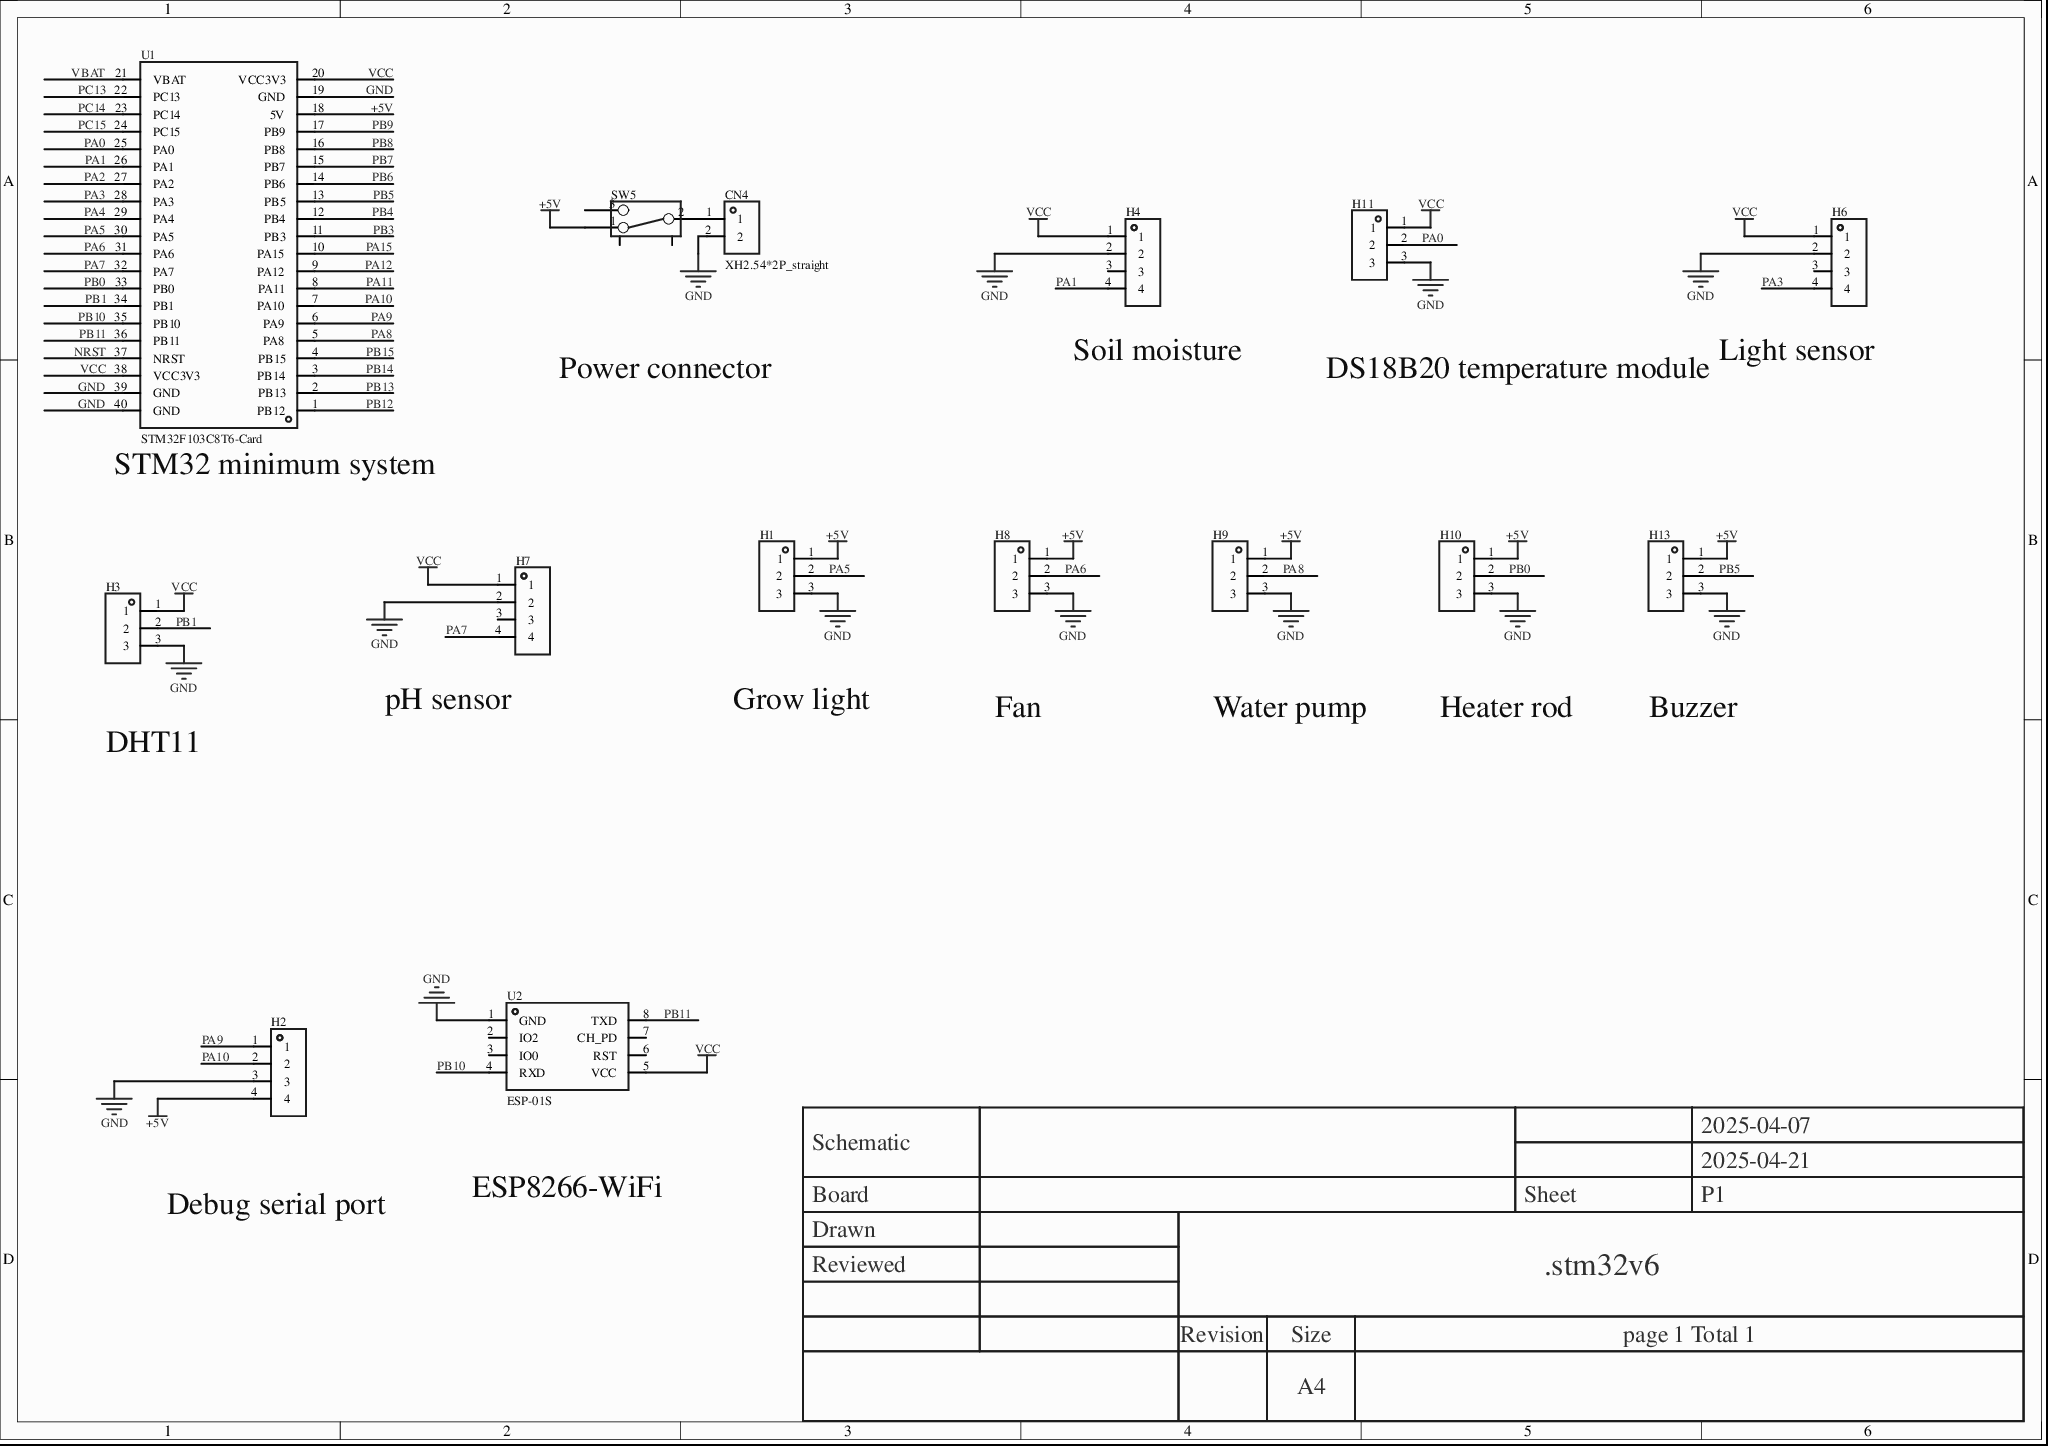
[diagram p0: MISC89003-3.schdoc]
# Altium project MISC89003-2.PrjPcb
1 sheet, 15 parts. Net scope: global (net labels, ports and power ports of the same name join across sheets).
Board file: MISC89003.pcbdoc

## Sheet MISC89003-3.schdoc
size 297 x 209 mm; Version: V1.0; @Project Name: MISC89003; @Page Count: 1; @Update Date: 2026-04-15; @Create Date: 2026-04-15; @Schematic Name: MISC89003; @Page No: 1; @Create Time: 23:22:16; @Update Time: 17:32:40; @Board Name: MISC89003

### Parts
CN4  XH2.54*2P_straight  [CONN-TH_2P-P2.50-XH2.54-2P]
H1  (no value)  [HDR-TH_3P-P2.54-V-F]
H2  (no value)  [HDR-TH_4P-P2.54-V-F]
H3  (no value)  [HDR-TH_3P-P2.54-V-F]
H4  (no value)  [HDR-TH_4P-P2.54-V-F]
H6  (no value)  [HDR-TH_4P-P2.54-V-F]
H7  (no value)  [HDR-TH_4P-P2.54-V-F]
H8  (no value)  [HDR-TH_3P-P2.54-V-F]
H9  (no value)  [HDR-TH_3P-P2.54-V-F]
H10  (no value)  [HDR-TH_3P-P2.54-V-F]
H11  (no value)  [HDR-TH_3P-P2.54-V-F]
H13  (no value)  [HDR-TH_3P-P2.54-V-F]
SW5  (no value)  [拨动开关]
U1  STM32F103C8T6-Card  [CONN-TH_L53.3-W22.9_STM32F103C8T6-CARD]
U2  ESP-01S  [WIFIM-TH_ESP-01S]

### Nets
+5V: H1.1 H2.4 H8.1 H9.1 H10.1 H13.1 SW5.1 U1.18(5V)
GND: CN4.2 H1.3 H2.3 H3.3 H4.2 H6.2 H7.2 H8.3 H9.3 H10.3 H11.3 H13.3 U1.19(GND) U1.39(GND) U1.40(GND) U2.1(GND)
VCC: H3.1 H4.1 H6.1 H7.1 H11.1 U1.20(VCC3V3) U1.38(VCC3V3) U2.5(VCC)
NRST: U1.37(NRST)
PA0: H11.2 U1.25(PA0)
PA1: H4.4 U1.26(PA1)
PA2: U1.27(PA2)
PA3: H6.4 U1.28(PA3)
PA4: U1.29(PA4)
PA5: H1.2 U1.30(PA5)
PA6: H8.2 U1.31(PA6)
PA7: H7.4 U1.32(PA7)
PA8: H9.2 U1.5(PA8)
PA9: H2.1 U1.6(PA9)
PA10: H2.2 U1.7(PA10)
PA11: U1.8(PA11)
PA12: U1.9(PA12)
PA15: U1.10(PA15)
PB0: H10.2 U1.33(PB0)
PB1: H3.2 U1.34(PB1)
PB3: U1.11(PB3)
PB4: U1.12(PB4)
PB5: H13.2 U1.13(PB5)
PB6: U1.14(PB6)
PB7: U1.15(PB7)
PB8: U1.16(PB8)
PB9: U1.17(PB9)
PB10: U1.35(PB10) U2.4(RXD)
PB11: U1.36(PB11) U2.8(TXD)
PB12: U1.1(PB12)
PB13: U1.2(PB13)
PB14: U1.3(PB14)
PB15: U1.4(PB15)
PC13: U1.22(PC13)
PC14: U1.23(PC14)
PC15: U1.24(PC15)
VBAT: U1.21(VBAT)
NetCN4_1: CN4.1 SW5.2

Not connected (* = marked no-connect by the designer): H4 3; H6 3; H7 3; SW5 3 4 5; U2 2(IO2)* 3(IO0)* 6(RST)* 7(CH_PD)*

### Notes on the sheet
- Power connector
- (near H4) Soil moisture
- DS18B20 temperature module
- (near H6) Light sensor
- (near U1) STM32 minimum system
- DHT11
- (near H7) pH sensor
- Grow light
- Fan
- Water pump
- Heater rod
- Buzzer
- Debug serial port
- ESP8266-WiFi
- 2025-04-07
- Schematic
- Board
- Sheet
- 2025-04-21
- P1
- Drawn
- Reviewed
- .stm32v6
- Revision
- Size
- A4
- page 1 Total 1

### Library data of the parts
CN4 = XH2.54*2P_直插: 3D Model: 325c595e30db4df8abe76612dd40b0fa0819f05c4eef4c71ace90d822a990e87; 3D Model Transform: 295.275,228.346,0,180,0,0,-0.002,-20.079,-137.795; AddInBom: yes; Device: XH2.54*2P_straight; Symbol: XH2.54*2P_straight; LCSC Part Name: XH2.54*2P_直插; Supplier Part: C9900008615; Manufacturer Part: XH2.54*2P_直插; Supplier Footprint: XH2.54_2P; JLCPCB Part Class: Extended Part; Supplier: LCSC; FootprintName: CONN-TH_2P-P2.50-XH2.54-2P; ConvertToPcb: yes; ModelName: CONN-TH_2P-P2.50-XH2.54-2P
H1 H3 H8-H11 H13 = HDR-F_2.54_1x3P: Symbol: PM254V-11-03-H85; 3D Model: f3b3cc5aae9641bf9e56fc160cef875b; 3D Model Transform: 299.9994,100,0,0,0,0,0,0,-118.11; ConvertToPcb: yes; ModelName: HDR2.54-F-LI-1X3P; Device: HDR-F_2.54_1x3P; Supplier Part: C541850; Supplier Footprint: 插件; FootprintName: HDR-TH_3P-P2.54-V-F; AddInBom: yes
H2 H4 = HDR-F_2.54_1x4P: Symbol: 2.54-1*4P female; ConvertToPcb: yes; ModelId: d187812051054f85879fcaa51a310d8e0819f05c4eef4c71ace90d822a990e87; ModelTransform: 419.6842,98.464,0,0,0,0,0,0,-118.11; Device: HDR-F_2.54_1x4P; FootprintName: HDR-TH_4P-P2.54-V-F; AddInBom: yes; SupplierPart: C2718488; Supplier Footprint: 插件; ModelName: HDR-TH_4P-P2.54-V-F
H6 H7 = HDR-F_2.54_1x4P: Symbol: 2.54-1*4P female; 3D Model: d187812051054f85879fcaa51a310d8e0819f05c4eef4c71ace90d822a990e87; 3D Model Transform: 419.6842,98.464,0,0,0,0,0,0,-118.11; ConvertToPcb: yes; Device: HDR-F_2.54_1x4P; Supplier Part: C2718488; Supplier Footprint: 插件; FootprintName: HDR-TH_4P-P2.54-V-F; AddInBom: yes; ModelName: HDR-TH_4P-P2.54-V-F
SW5 = 拨动开关_正: Device: Toggle switch_positive; Symbol: Toggle switch; ConvertToPcb: yes; ModelId: 4321fe59a4074cbfb4989553f297c68f0819f05c4eef4c71ace90d822a990e87; ModelName: SW-TH_SS-12D02-VG4; ModelTransform: 370.09,208.7,472.35,0,0,0,0,0,-110; FootprintName: Toggle switch; AddInBom: yes; Supplier Footprint: 插件
U1 = STM32F103C8T6-Card: AddInBom: yes; Device: STM32F103C8T6-Card; Symbol: STM32F103C8T6-CARD; FootprintName: CONN-TH_L53.3-W22.9_STM32F103C8T6-CARD; LCSC Part Name: STM32F103C8T6-Card; SupplierPart: C9900077949; ManufacturerPart: STM32F103C8T6-Card; Supplier Footprint: 插件; Supplier: LCSC; ConvertToPcb: yes
U2 = ESP-01S_C111009: 3D Model: eb7175da78ae48b3b1568cfe3027405f0819f05c4eef4c71ace90d822a990e87; 3D Model Transform: 582.676,976.37608,0,0,0,0,0,388.346,-118.11; AddInBom: yes; Symbol: ESP-01S; Device: ESP-01S_C111009; LCSC Part Name: ESP-01S; Supplier Part: C111009; Manufacturer Part: ESP-01S; Supplier Footprint: -; JLCPCB Part Class: Extended Part; Supplier: LCSC; ConvertToPcb: yes; FootprintName: WIFIM-TH_ESP-01S; ModelName: WIFIM-TH_ESP-01S